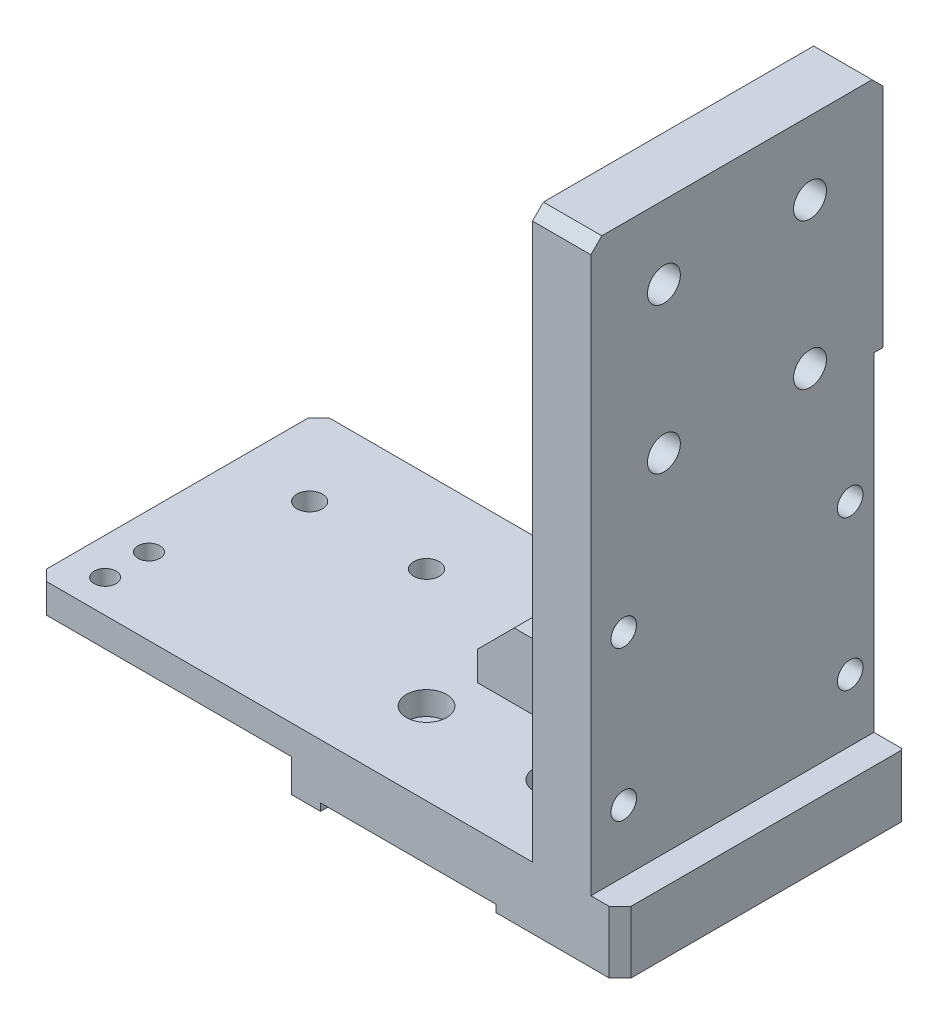
from build123d import *

# Parameters (mm, degrees)
EXTRUDE_2_DEPTH              = 40
SKETCH_4_W                   = 2.5
SKETCH_4_H                   = 90
CUT_EXTRUDE_2_DEPTH          = 80
EXTRUDE_3_DEPTH              = 5
FILLET_1_R                   = 10
CHAMFER_1_SIZE               = 10
HOLE_WIZARD_M6_1_D           = 6.6
HOLE_WIZARD_M6_1_CBORE_D     = 11
HOLE_WIZARD_M6_1_CBORE_DEPTH = 6.4
CHAMFER_2_SIZE               = 3
HOLE_WIZARD_7_0_7_1_D        = 7
HOLE_WIZARD_M8_2_D           = 9
HOLE_WIZARD_M8_2_CBORE_D     = 15
HOLE_WIZARD_M8_2_CBORE_DEPTH = 8.6
SKETCH_16_W                  = 163.711624667
SKETCH_16_H                  = 2.5
CUT_EXTRUDE_3_DEPTH          = 179.955301682
SKETCH_17_W                  = 70
SKETCH_17_H                  = 9
CUT_EXTRUDE_4_DEPTH          = 198.834526815
CHAMFER_4_SIZE               = 3
HOLE_WIZARD_7_0_7_2_D        = 7
HOLE_WIZARD_6_0_6_1_D        = 6


with BuildPart() as part:
    # 草图2 → 凸台-拉伸2 (new, symmetric)
    with BuildSketch(Plane.XY):
        Polygon((46, -8.5), (80, -8.5), (80, 8.5), (72, 8.5), (72, 163.5), (56, 163.5), (56, 8.5), (-80, 8.5), (-80, -8.5), (-2, -8.5), (-2, -6.5), (46, -6.5), align=None)
    extrude(amount=EXTRUDE_2_DEPTH, both=True)

    # 草图4 → 切除-拉伸2 (cut)
    with BuildSketch(Plane.ZY.offset(-56)):
        with Locations((-38.75, 53.5)):
            Rectangle(SKETCH_4_W, SKETCH_4_H)
    extrude(amount=-CUT_EXTRUDE_2_DEPTH, mode=Mode.SUBTRACT)

    # 草图5 → 凸台-拉伸3 (add, symmetric)
    with BuildSketch(Plane.XY):
        Polygon((46, 8.5), (6, 8.5), (6, 26.5), (38, 26.5), (38, 83.5), (56, 83.5), (56, 18.5), align=None)
    extrude(amount=EXTRUDE_3_DEPTH, both=True)

    # 圆角1
    fillet_1_edges = [part.edges().sort_by_distance(p)[0] for p in [
        (38, 26.5, 0),
    ]]
    fillet(fillet_1_edges, radius=FILLET_1_R)

    # 倒角1
    chamfer_1_edges = [part.edges().sort_by_distance(p)[0] for p in [
        (6, 26.5, 0),
        (38, 83.5, 0),
    ]]
    chamfer(chamfer_1_edges, length=CHAMFER_1_SIZE)

    # M6 六角凹头螺钉的柱形沉头孔1 (through all)
    with Locations(Plane(origin=(0, 8.5, 0), x_dir=(1, 0, 0), z_dir=(0, 1, 0))):
        with Locations((4.5, 17.5), (39.5, 17.5), (39.5, -17.5), (4.5, -17.5)):
            CounterBoreHole(HOLE_WIZARD_M6_1_D / 2, HOLE_WIZARD_M6_1_CBORE_D / 2, HOLE_WIZARD_M6_1_CBORE_DEPTH)

    # 倒角2
    chamfer_2_edges = [part.edges().sort_by_distance(p)[0] for p in [
        (64, 163.5, 40),
        (64, 163.5, -40),
        (80, 0, -40),
        (-80, 0, 40),
        (80, 0, 40),
    ]]
    chamfer(chamfer_2_edges, length=CHAMFER_2_SIZE)

    # Ø7.0 (7) 直径孔1 (through all)
    with Locations(Plane.ZY.offset(-56)):
        with Locations((-31, 25.5), (-31, 66.5), (31, 66.5), (31, 25.5)):
            Hole(HOLE_WIZARD_7_0_7_1_D / 2)

    # M8 六角凹头螺钉的柱形沉头孔2 (through all)
    with Locations(Plane.ZY.offset(-56)):
        with Locations((-20, 143.5), (-20, 103.5), (20, 103.5), (20, 143.5)):
            CounterBoreHole(HOLE_WIZARD_M8_2_D / 2, HOLE_WIZARD_M8_2_CBORE_D / 2, HOLE_WIZARD_M8_2_CBORE_DEPTH)

    # 草图16 → 切除-拉伸3 (cut, through all)
    with BuildSketch(Plane(origin=(0, 8.5, 0), x_dir=(1, 0, 0), z_dir=(0, 1, 0))):
        with Locations((-1.855812334, 38.75)):
            Rectangle(SKETCH_16_W, SKETCH_16_H)
    extrude(amount=-CUT_EXTRUDE_3_DEPTH, mode=Mode.SUBTRACT)

    # 草图17 → 切除-拉伸4 (cut, through all)
    with BuildSketch(Plane(origin=(0, 0, -37.5), x_dir=(-1, 0, 0), z_dir=(0, 0, -1))):
        with Locations((45, -4)):
            Rectangle(SKETCH_17_W, SKETCH_17_H)
    extrude(amount=-CUT_EXTRUDE_4_DEPTH, mode=Mode.SUBTRACT)

    # 倒角4
    chamfer_4_edges = [part.edges().sort_by_distance(p)[0] for p in [
        (-80, 4.5, -37.5),
    ]]
    chamfer(chamfer_4_edges, length=CHAMFER_4_SIZE)

    # Ø7.0 (7) 直径孔2 (through all)
    with Locations(Plane(origin=(0, 8.5, 0), x_dir=(1, 0, 0), z_dir=(0, 1, 0))):
        with Locations((-28, 15), (-60, 15)):
            Hole(HOLE_WIZARD_7_0_7_2_D / 2)

    # Ø6.0 (6) 直径孔1 (through all)
    with Locations(Plane(origin=(0, 8.5, 0), x_dir=(1, 0, 0), z_dir=(0, 1, 0))):
        with Locations((-70, -31), (-70, -19)):
            Hole(HOLE_WIZARD_6_0_6_1_D / 2)


solid = part.part
